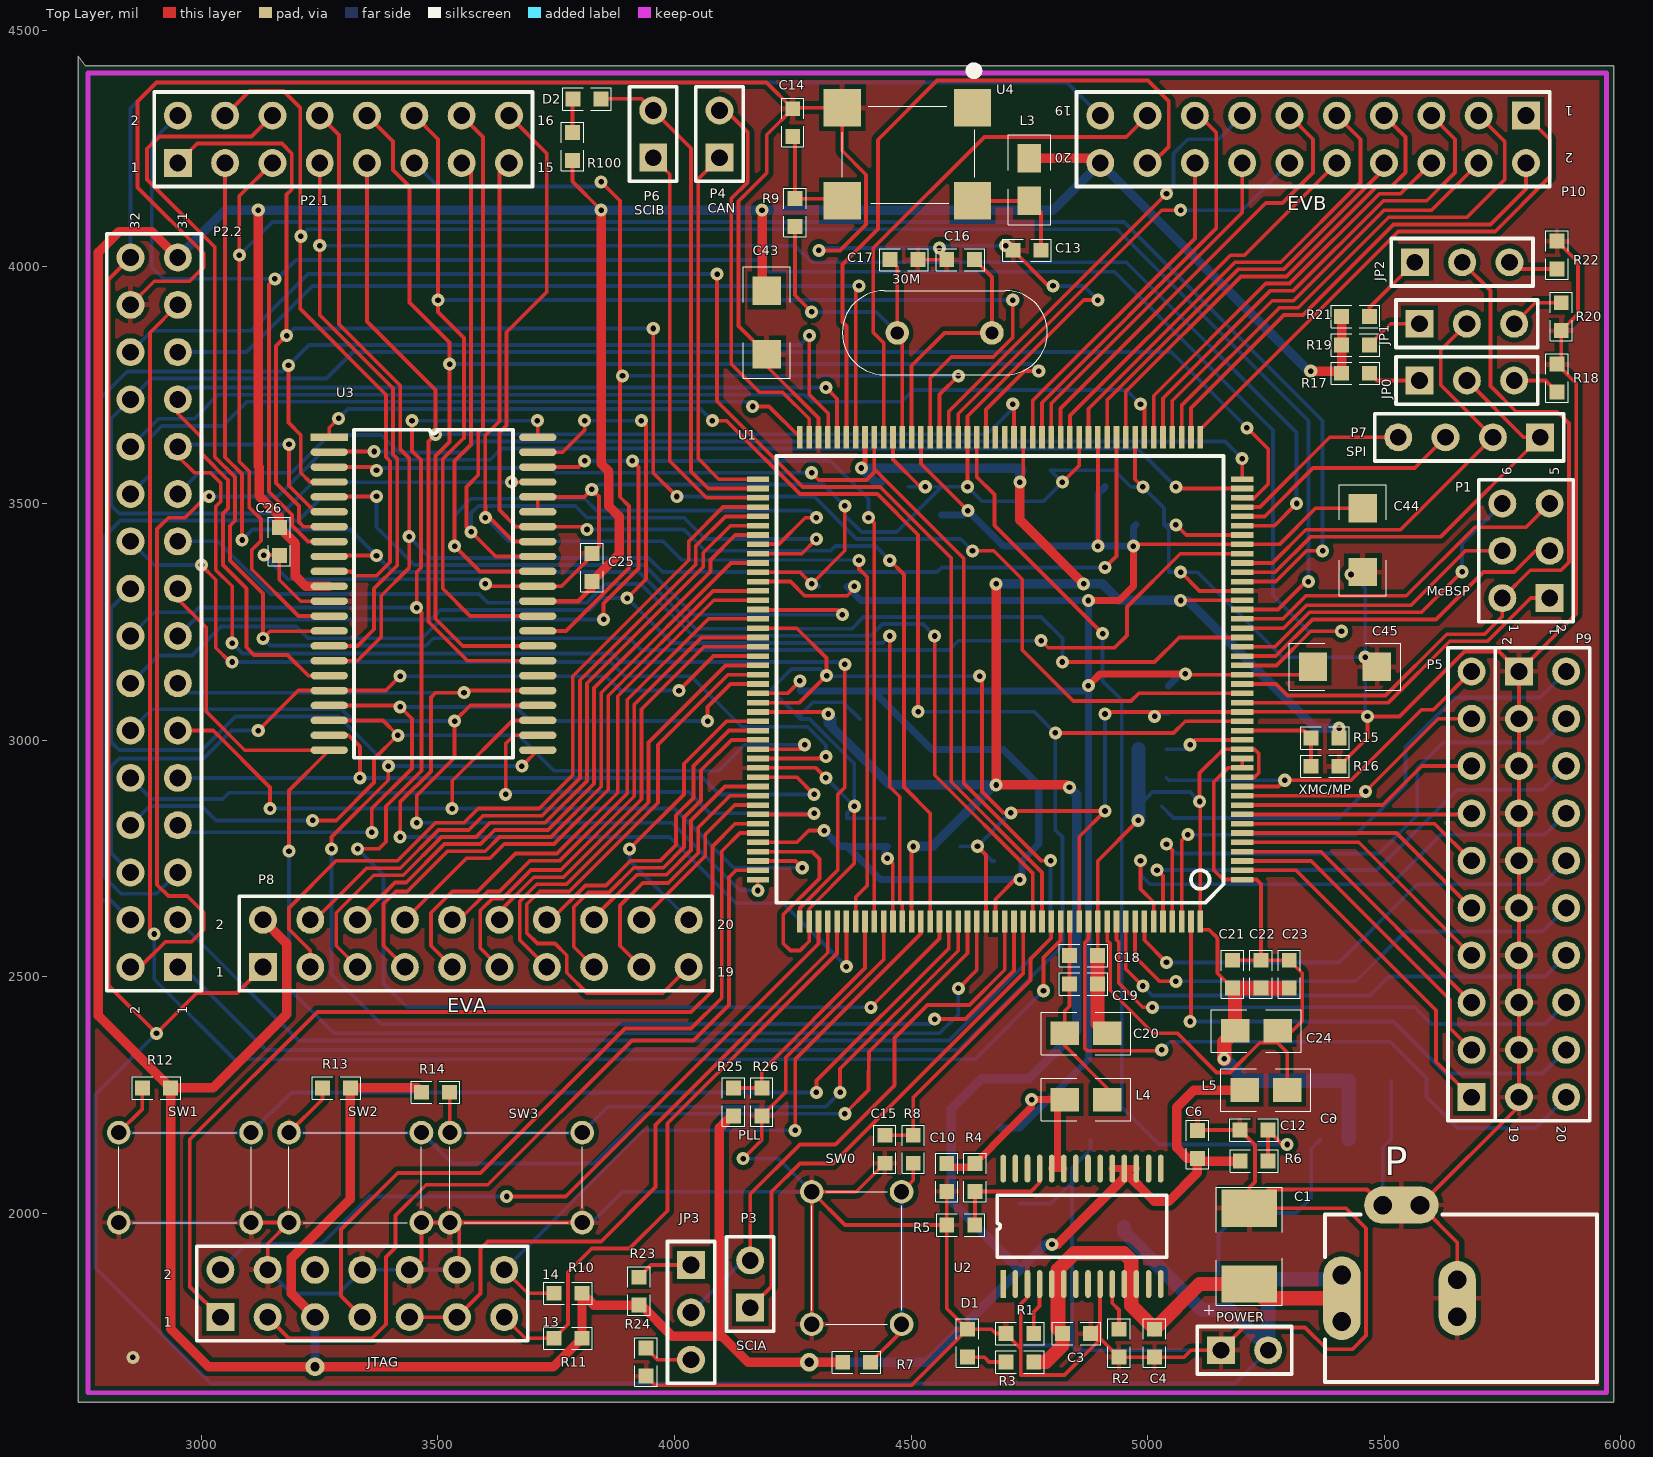
[diagram p0: Top Layer view]
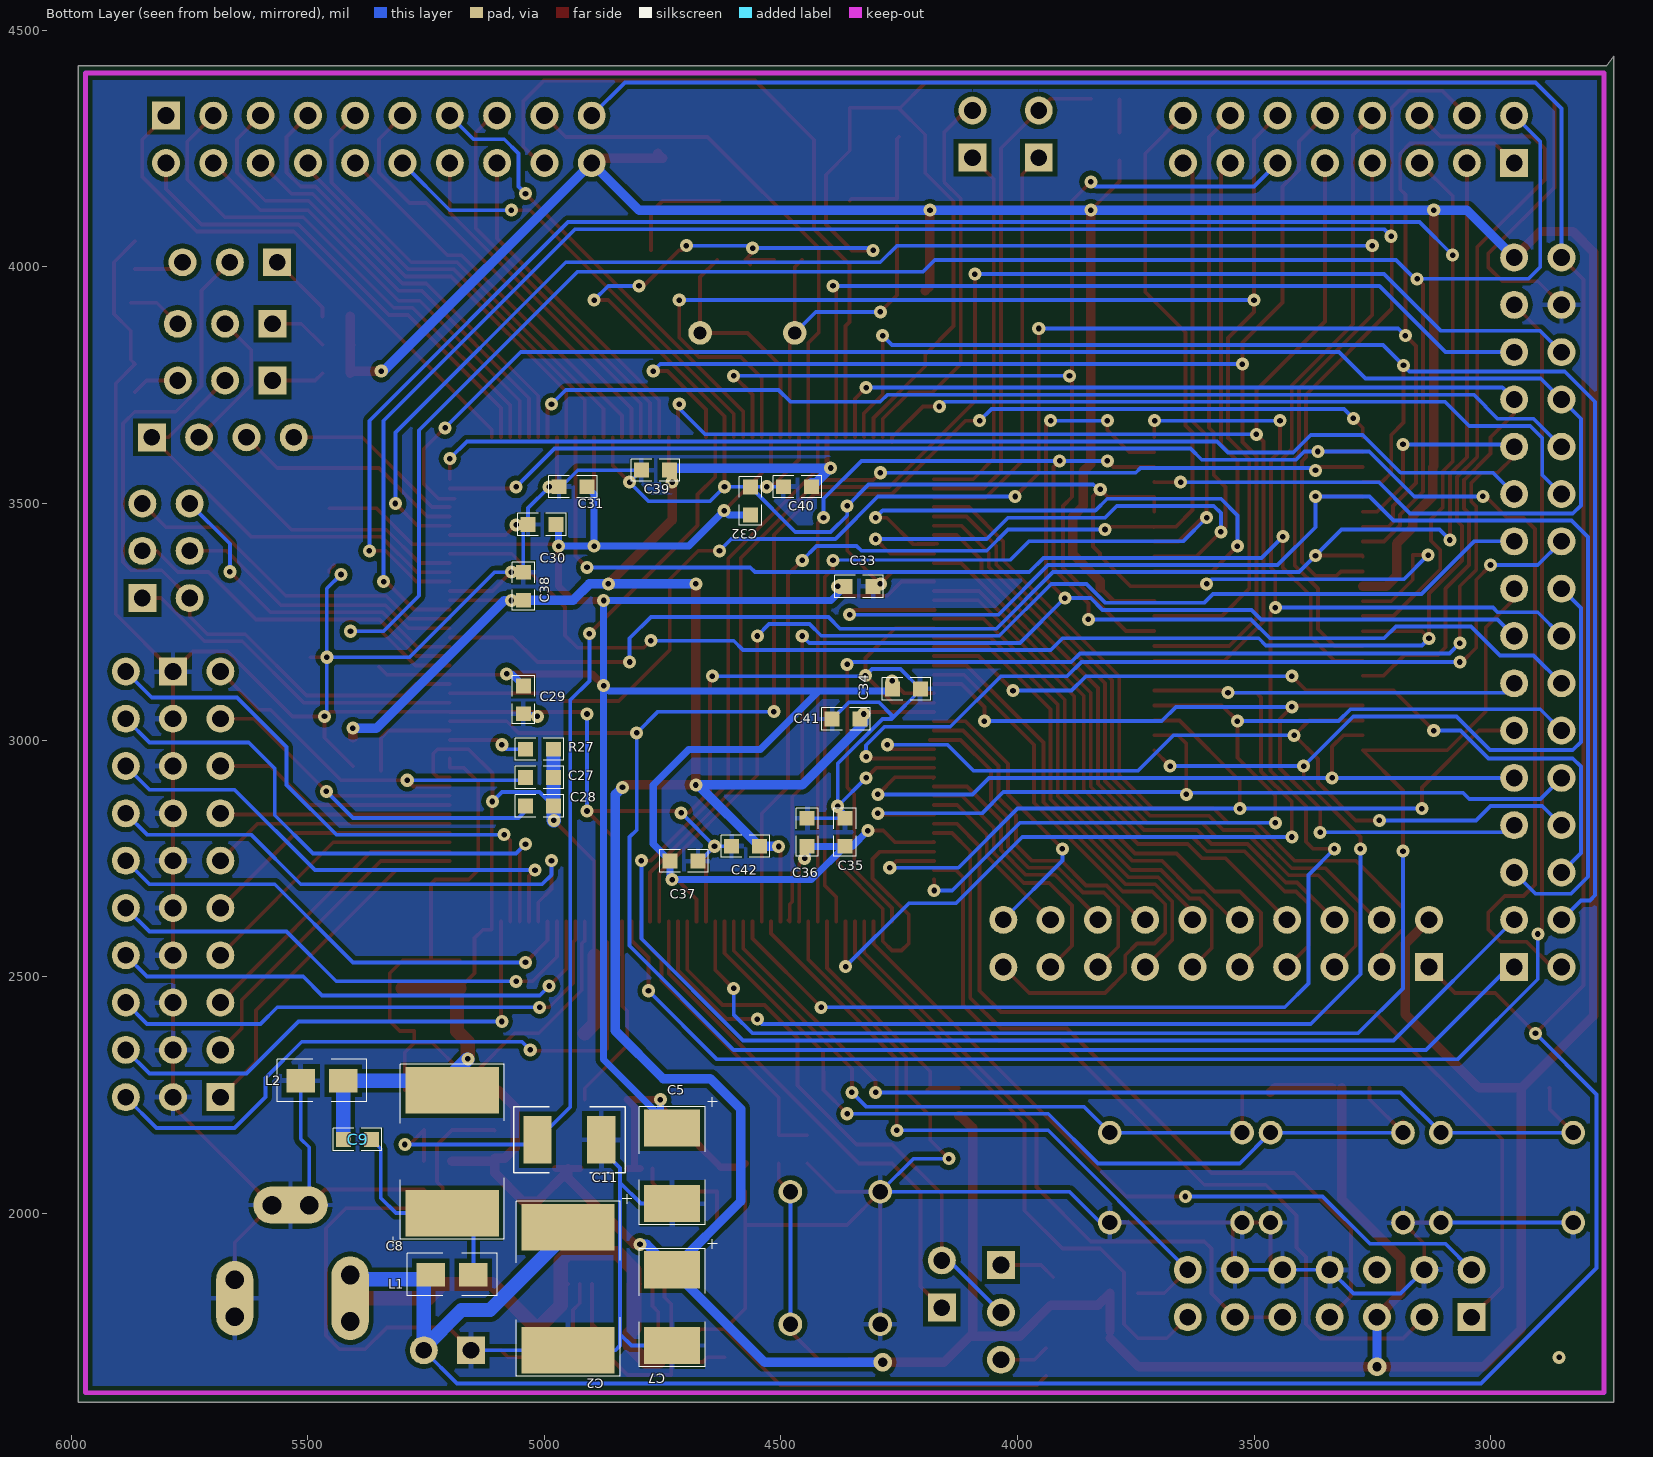
[diagram p1: Bottom Layer view, seen from below]
# Altium PCB MISC76198.PCBDOC (part 1 of 2)
Units mil, origin at the board's own origin, x right, y up, seen from the top; angles counter-clockwise.
Board outline 3245 x 2845 mil, 2 copper layers (Top Layer, Bottom Layer); 107 components, 158 nets, 601 pads, 196 vias.

## Layer stack, top to bottom (the 12.6 mil dielectric is the usual default, probably not edited)
Top Layer: signal copper 1.4
Dielectric: dielectric 12.6, FR-4, Dk 4.8
Bottom Layer: signal copper 1.4

## Board outline
2755,4425 5985,4425 5985,1600 2740,1600 2740,4445

## Design rules (kind name [scope] priority, off if disabled: settings)
Clearance [All] p1: gap=7
ComponentClearance [All] p1: gap=10 collisioncheckmode=0
PolygonConnect [All] p1: connectstyle=Relief reliefconductorwidth=10 reliefentries=4 polygonreliefangle="90 Angle"
RoutingVias [All] p1: holewidth=11.81 width=27.56 viastyle="Through Hole" minholewidth=11 minwidth=27 maxholewidth=39.37 maxwidth=39.37
SolderMaskExpansion [All] p1: expansion=4
TestPointUsage [All] p1: valid=0 allowmultiple=FALSE
Testpoint [All] p1: side=15 testpointundercomponent=TRUE minsize=40 maxsize=100 preferedsize=60 minholesize=0 maxholesize=40 preferedholesize=32 testpointgrid=1 style=1023 order=-539222988
Width Width_2 [InNet('3.3V')] p1: maxlimit=30 minlimit=8 preferedwidth=10 toplayer_prefwidth=8 bottomlayer_prefwidth=20 minimp=50.000000 maximp=50.000000 favimp=50.000000
Width Width_1 [InNet('1.8V')] p2: maxlimit=30 minlimit=8 preferedwidth=10 toplayer_prefwidth=8 bottomlayer_prefwidth=15 minimp=50.000000 maximp=50.000000 favimp=50.000000
Width [All] p3: maxlimit=39.37 minlimit=8 preferedwidth=10 toplayer_prefwidth=8 bottomlayer_prefwidth=8 minimp=50.000000 maximp=50.000000 favimp=50.000000
17 further rules are at their usual default settings.

## Components (designator, comment, footprint, x,y, rotation, side; value= is the part's Value field where it differs from the comment)
30M "XTAL" TXAL 4570,3900 r90 top
C1 "Cap Pol1" C2 5375,1810 r90 top
C2 "Cap Pol1" C1 5035,1910 r270 bottom
C3 "Cap" 0603 4895,1750 r0 top
C4 "Cap" 0603 5010,1770 r90 top
C5 "Cap Pol1" C2 4890,2220 r270 bottom
C6 "Cap" 0603 5110,2100 r270 top
C7 "Cap Pol1" c2 4890,1920 r270 bottom
C8 "Cap Pol1" C1 5110,2060 r90 bottom
C9 "Cap" 0603 5350,2160 r180 bottom
C10 "Cap" 0603 4580,2030 r270 top
C11 "Cap Pol1" 1210 4950,2160 r180 bottom
C12 "Cap" 0603 5270,2180 r0 top
C13 "Cap" 0603 4790,4040 r0 top
C14 "Cap" 0603 4254.56,4260 r270 top
C15 "Cap" 0603 4440,2180 r90 top
C16 "Cap Semi" 0603 4650,4020 r0 top
C17 "Cap Semi" 0603 4530,4020 r0 top
C18 "Cap Semi" 0603 4819.61,2540 r180 top
C19 "Cap Semi" 0603 4819.61,2480 r180 top
C20 "Cap Pol1" 0805 4930,2380 r0 top
C21 "Cap Semi" 0603 5175,2550 r90 top
C22 "Cap Semi" 0603 5235,2550 r90 top
C23 "Cap Semi" 0603 5295,2550 r90 top
C24 "Cap Pol1" 0805 5170,2385 r180 top
C25 "Cap" 0603 3830,3320 r270 top
C26 "Cap" 0603 3160,3465 r90 top
C27 "Cap" 0603 4965,2925 r180 bottom
C28 "Cap" 0603 4965,2865 r180 bottom
C29 "0.1uF" 0603 5040,3040 r270 bottom
C30 "0.1uF" 0603 4960,3460 r180 bottom
C31 "0.1uF" 0603 4894.88,3540 r180 bottom
C32 "0.1uF" 0603 4560,3460 r270 bottom
C33 "0.1uF" 0603 4380,3320 r0 bottom
C34 "0.1uF" 0603 4280,3103.69 r0 bottom
C35 "0.1uF" 0603 4360,2760 r270 bottom
C36 "0.1uF" 0603 4440,2760 r270 bottom
C37 "0.1uF" 0603 4750,2740 r0 bottom
C38 "0.1uF" 0603 5040,3280 r270 bottom
C39 "0.1uF" 0603 4720,3575 r180 bottom
C40 "0.1uF" 0603 4420,3540 r180 bottom
C41 "0.1uF" 0603 4407.44,3040 r0 bottom
C42 "0.1uF" 0603 4530,2780 r180 bottom
C43 "Cap Pol1" 1206 4200,3900 r270 top
C44 "Cap Pol1" 1206 5460,3440 r270 top
C45 "Cap Pol1" 1206 5400,3160 r0 top
D1 "RED" 0603 4615,1770 r90 top
D2 "RED" 0603 3860,4360 r0 top
JP0 "BOOT0" HDR1X3 5575,3760 r0 top (schematic designator JP2)
JP1 "BOOT1" HDR1X3 5575,3880 r0 top (schematic designator JP3)
JP2 "BOOT2" HDR1X3 5565,4010 r0 top (schematic designator JP4)
JP3 "BOOT3" HDR1X3 4035,1890 r270 top (schematic designator JP5)
JTAG "Header 7X2" HDR2X7 3040,1780 r0 top
L1 "Inductor" 0805 5135,1870 r180 bottom
L2 "Inductor" 0805 5410,2280 r180 bottom
L3 "Inductor" 0805 4750.08,4244.85 r90 top
L4 "Inductor" 0805 4930,2240 r0 top
L5 "Inductor" 0805 5190,2260 r180 top
P "PWR2.5" KLD-0202 5950,1820 r180 top
P1 "MCBSP" HDR2X3 5850,3300 r90 top
P2.1 "Header 8X2" HDR2X8 2950,4220 r0 top
P2.2 "Header 16X2" HDR2X16 2950,2520 r90 top (schematic designator P2.3)
P3 "SCIA" HDR1X2 4160,1800 r90 top
P4 "SCIB" HDR1X2 4095,4231 r90 top
P5 "Header 10" HDR1X10 5685,2245 r90 top
P6 "CAN" HDR1X2 3955,4231 r90 top
P7 "SPI" HDR1X4 5830,3640 r180 top
P8 "Header 10X2" HDR2X10 3130,2520 r0 top
P9 "Header 10X2" HDR2X10 5785,3145 r270 top
P10 "Header 10X2" HDR2X10 5800,4320 r180 top
POWER "Header 2" HDR1X2 5155,1710 r0 top
R1 "Res2" 0603 4775,1750 r0 top
R2 "Res2" 0603 4935,1770 r90 top
R3 "Res2" 0603 4775,1690 r0 top
R4 "Res2" 0603 4640,2030 r270 top
R5 "Res2" 0603 4560,1970 r180 top
R6 "Res2" 0603 5180.39,2105.44 r180 top
R7 "1.5K" 0603 4340,1680 r180 top
R8 "100" 0603 4500,2180 r90 top
R9 "1k" 0603 4250,4160 r90 top
R10 "Res2" 0603 3820,1835 r0 top
R11 "Res2" 0603 3820,1740 r0 top
R12 "Res2" 0603 2860,2260 r180 top
R13 "Res2" 0603 3240,2260 r180 top
R14 "Res2" 0603 3540,2260 r0 top
R15 "10K" 0603 5330,3000 r180 top
R16 "1k" 0603 5330,2940 r180 top
R17 "10K" 0603 5485,3780 r0 top
R18 "2.2K" 0603 5870,3720 r270 top
R19 "10K" 0603 5485,3840 r0 top
R20 "2.2K" 0603 5870,3940 r90 top
R21 "10k" 0603 5485,3900 r0 top
R22 "2.2K" 0603 5870,3980 r270 top
R23 "10k" 0603 3920,1880 r90 top
R24 "2.2K" 0603 3935,1730 r90 top
R25 "10k" 0603 4120,2280 r90 top
R26 "2.2K" 0603 4180,2280 r90 top
R27 "24.9K" 0603 4965,2985 r180 bottom
R100 "Res2" 0603 3780,4300 r90 top
SW0 "KEY4" key 4280,2060 r0 top (schematic designator SW1)
SW1 "KEY4" key 3120,2180 r270 top (schematic designator SW4)
SW2 "KEY4" key 3480,2180 r270 top (schematic designator SW3)
SW3 "KEY4" key 3820,2180 r270 top (schematic designator SW2)
U1 "TMS320F2812" QFP176 5200,2705 r90 top locked
U2 "TPS767D301" TSOP28(0.65mm) 4695,1850 r90 top
U3 "CY7C1041CV    SDRAM" TSOP44(0.8mm) 3270,3640 r0 top
U4 "30M" CRYSTAL1 4630,4140 r180 top

## Footprints (in the part's own frame and the unit in brackets; to place one, negate y for a bottom-side part, rotate by r counter-clockwise, add the part's x,y. Pads: shape width x height; smd on the part's side, far side on the other; paste and mask are expansions set on the pad)
0603 [mm]
  rect 0.8x0.8 smd: 1(-1.895,-0.116) 2(-0.395,-0.116)
  silkscreen extent -2.45,-0.72 0.15,0.48
0805 [mil]
  rect 60x50 smd: 1(-105.15,-0.08) 2(-15.15,-0.08)
  silkscreen extent -155,-45 35,45
1206 [mil]
  rect 60x60 smd: 1(-50.17,-5) 2(84.83,-5)
  silkscreen extent -100,-55 135,45
1210 [mil]
  rect 60x100 smd: 1(-64.65,-5.12) 2(70.35,-5.12)
  silkscreen extent -115,-75 120,65
C1 [mm]
  rect 2.5x5 smd: 1(-1.524,2.159) 2(5.08,2.159)
  silkscreen extent -3.3,-0.64 6.48,5.59
C2 [mm]
  rect 2x3 smd: 1(1.016,4.064) 2(5.08,4.064)
  silkscreen extent -0.64,2.29 6.22,6.48
c2 [mm]
  rect 2x3 smd: 1(1.016,4.064) 2(5.08,4.064)
  silkscreen extent -0.63,2.29 6.22,6.48
CRYSTAL1 [mm]
  rect 2x2 smd: 1(0,-5) 2(7,-5) 3(7,0) 4(0,0)
  silkscreen extent -0.27,-7.18 6.98,0.13
HDR1X2 [mm] "Connector; Header; 2 Position"
  rect 1.5x1.5 hole 0.9: 1(0,0)
  round 1.5 hole 0.9: 2(2.54,0)
  silkscreen extent -1.27,-1.27 3.81,1.27
HDR1X3 [mm] "Connector; Header; 3 Position"
  rect 1.5x1.5 hole 0.9: 1(0,0)
  round 1.5 hole 0.9: 2(2.54,0) 3(5.08,0)
  silkscreen extent -1.27,-1.27 6.35,1.27
HDR1X4 [mm] "Connector; Header; 4 Position"
  rect 1.5x1.5 hole 0.9: 1(0,0)
  round 1.5 hole 0.9: 2(2.54,0) 3(5.08,0) 4(7.62,0)
  silkscreen extent -1.27,-1.27 8.89,1.27
HDR1X10 [mm] "Connector; Header; 10 Position"
  rect 1.5x1.5 hole 0.9: 1(0,0)
  round 1.5 hole 0.9: 2(2.54,0) 3(5.08,0) 4(7.62,0) 5(10.16,0) 6(12.7,0) 7(15.24,0) 8(17.78,0) 9(20.32,0) 10(22.86,0)
  silkscreen extent -1.27,-1.27 24.13,1.27
HDR2X3 [mm] "Connector; Header; 3x2 Position"
  rect 1.5x1.5 hole 0.9: 1(0,0)
  round 1.5 hole 0.9: 2(0,2.54) 3(2.54,0) 4(2.54,2.54) 5(5.08,0) 6(5.08,2.54)
  silkscreen extent -1.27,-1.27 6.35,3.81
HDR2X7 [mm] "Connector; Header; 7x2 Position"
  rect 1.5x1.5 hole 0.9: 1(0,0)
  round 1.5 hole 0.9: 2(0,2.54) 3(2.54,0) 4(2.54,2.54) 5(5.08,0) 6(5.08,2.54) 7(7.62,0) 8(7.62,2.54) 9(10.16,0) 10(10.16,2.54) 11(12.7,0) 12(12.7,2.54) 13(15.24,0) 14(15.24,2.54)
  silkscreen extent -1.27,-1.27 16.51,3.81
HDR2X8 [mm] "Connector; Header; 8x2 Position"
  rect 1.5x1.5 hole 0.9: 1(0,0)
  round 1.5 hole 0.9: 2(0,2.54) 3(2.54,0) 4(2.54,2.54) 5(5.08,0) 6(5.08,2.54) 7(7.62,0) 8(7.62,2.54) 9(10.16,0) 10(10.16,2.54) 11(12.7,0) 12(12.7,2.54) 13(15.24,0) 14(15.24,2.54) 15(17.78,0) 16(17.78,2.54)
  silkscreen extent -1.27,-1.27 19.05,3.81
HDR2X10 [mm] "Connector; Header; 10x2 Position"
  rect 1.5x1.5 hole 0.9: 1(0,0)
  round 1.5 hole 0.9: 2(0,2.54) 3(2.54,0) 4(2.54,2.54) 5(5.08,0) 6(5.08,2.54) 7(7.62,0) 8(7.62,2.54) 9(10.16,0) 10(10.16,2.54) 11(12.7,0) 12(12.7,2.54) 13(15.24,0) 14(15.24,2.54) 15(17.78,0) 16(17.78,2.54) 17(20.32,0) 18(20.32,2.54) 19(22.86,0) 20(22.86,2.54)
  silkscreen extent -1.27,-1.27 24.13,3.81
HDR2X16 [mm] "Connector; Header; 16x2 Position"
  rect 1.5x1.5 hole 0.9: 1(0,0)
  round 1.5 hole 0.9: 2(0,2.54) 3(2.54,0) 4(2.54,2.54) 5(5.08,0) 6(5.08,2.54) 7(7.62,0) 8(7.62,2.54) 9(10.16,0) 10(10.16,2.54) 11(12.7,0) 12(12.7,2.54) 13(15.24,0) 14(15.24,2.54) 15(17.78,0) 16(17.78,2.54) 17(20.32,0) 18(20.32,2.54) 19(22.86,0) 20(22.86,2.54) 21(25.4,0) 22(25.4,2.54) 23(27.94,0) 24(27.94,2.54) 25(30.48,0) 26(30.48,2.54) 27(33.02,0) 28(33.02,2.54) 29(35.56,0) 30(35.56,2.54) 31(38.1,0) 32(38.1,2.54)
  silkscreen extent -1.27,-1.27 39.37,3.81
key [mil]
  round 50 hole 32: 1(10,-15) 2(10,-295) 3(200,-15) 4(200,-295)
  silkscreen extent 10,-295 200,-15
KLD-0202 [mm] "DC Power Jack, 2.5mm, KLD Series, PCB Mount"
  oval 2x4.5 all layers, no hole: 1(13.7,0)
  round 1.5 hole 1: 1A(13.7,-1.25) 1B(13.7,1.25) 2A(7.5,-1) 2B(7.5,1) 3A(9.5,-5) 3B(11.5,-5)
  oval 2x4 all layers, no hole: 2(7.5,0)
  oval 4x2 all layers, no hole: 3(10.5,-5)
  silkscreen extent 0,-4.5 14.6,4.5
QFP176 [mm]
  rect 0.3x1.2 smd: 1(0,0) 2(0.5,0) 3(1,0) 4(1.5,0) 5(2,0) 6(2.5,0) 7(3,0) 8(3.5,0) 9(4,0) 10(4.5,0) 11(5,0) 12(5.5,0) 13(6,0) 14(6.5,0) 15(7,0) 16(7.5,0) 17(8,0) 18(8.5,0) 19(9,0) 20(9.5,0) 21(10,0) 22(10.5,0) 23(11,0) 24(11.5,0) 25(12,0) 26(12.5,0) 27(13,0) 28(13.5,0) 29(14,0) 30(14.5,0) 31(15,0) 32(15.5,0) 33(16,0) 34(16.5,0) 35(17,0) 36(17.5,0) 37(18,0) 38(18.5,0) 39(19,0) 40(19.5,0) 41(20,0) 42(20.5,0) 43(21,0) 44(21.5,0) 89(21.5,26) 90(21,26) 91(20.5,26) 92(20,26) 93(19.5,26) 94(19,26) 95(18.5,26) 96(18,26) 97(17.5,26) 98(17,26) 99(16.5,26) 100(16,26) 101(15.5,26) 102(15,26) 103(14.5,26) 104(14,26) 105(13.5,26) 106(13,26) 107(12.5,26) 108(12,26) 109(11.5,26) 110(11,26) 111(10.5,26) 112(10,26) 113(9.5,26) 114(9,26) 115(8.5,26) 116(8,26) 117(7.5,26) 118(7,26) 119(6.5,26) 120(6,26) 121(5.5,26) 122(5,26) 123(4.5,26) 124(4,26) 125(3.5,26) 126(3,26) 127(2.5,26) 128(2,26) 129(1.5,26) 130(1,26) 131(0.5,26) 132(0,26)
  rect 1.2x0.3 smd: 45(23.75,2.25) 46(23.75,2.75) 47(23.75,3.25) 48(23.75,3.75) 49(23.75,4.25) 50(23.75,4.75) 51(23.75,5.25) 52(23.75,5.75) 53(23.75,6.25) 54(23.75,6.75) 55(23.75,7.25) 56(23.75,7.75) 57(23.75,8.25) 58(23.75,8.75) 59(23.75,9.25) 60(23.75,9.75) 61(23.75,10.25) 62(23.75,10.75) 63(23.75,11.25) 64(23.75,11.75) 65(23.75,12.25) 66(23.75,12.75) 67(23.75,13.25) 68(23.75,13.75) 69(23.75,14.25) 70(23.75,14.75) 71(23.75,15.25) 72(23.75,15.75) 73(23.75,16.25) 74(23.75,16.75) 75(23.75,17.25) 76(23.75,17.75) 77(23.75,18.25) 78(23.75,18.75) 79(23.75,19.25) 80(23.75,19.75) 81(23.75,20.25) 82(23.75,20.75) 83(23.75,21.25) 84(23.75,21.75) 85(23.75,22.25) 86(23.75,22.75) 87(23.75,23.25) 88(23.75,23.75) 133(-2.25,23.75) 134(-2.25,23.25) 135(-2.25,22.75) 136(-2.25,22.25) 137(-2.25,21.75) 138(-2.25,21.25) 139(-2.25,20.75) 140(-2.25,20.25) 141(-2.25,19.75) 142(-2.25,19.25) 143(-2.25,18.75) 144(-2.25,18.25) 145(-2.25,17.75) 146(-2.25,17.25) 147(-2.25,16.75) 148(-2.25,16.25) 149(-2.25,15.75) 150(-2.25,15.25) 151(-2.25,14.75) 152(-2.25,14.25) 153(-2.25,13.75) 154(-2.25,13.25) 155(-2.25,12.75) 156(-2.25,12.25) 157(-2.25,11.75) 158(-2.25,11.25) 159(-2.25,10.75) 160(-2.25,10.25) 161(-2.25,9.75) 162(-2.25,9.25) 163(-2.25,8.75) 164(-2.25,8.25) 165(-2.25,7.75) 166(-2.25,7.25) 167(-2.25,6.75) 168(-2.25,6.25) 169(-2.25,5.75) 170(-2.25,5.25) 171(-2.25,4.75) 172(-2.25,4.25) 173(-2.25,3.75) 174(-2.25,3.25) 175(-2.25,2.75) 176(-2.25,2.25)
  silkscreen extent -1.25,1 22.75,25
TSOP28(0.65mm) [mm]
  rect 1.5x0.3 smd: 1(0,0)
  oval 1.5x0.3 smd: 2(0,-0.65) 3(0,-1.3) 4(0,-1.95) 5(0,-2.6) 6(0,-3.25) 7(0,-3.9) 8(0,-4.55) 9(0,-5.2) 10(0,-5.85) 11(0,-6.5) 12(0,-7.15) 13(0,-7.8) 14(0,-8.45) 15(6.2,-8.45) 16(6.2,-7.8) 17(6.2,-7.15) 18(6.2,-6.5) 19(6.2,-5.85) 20(6.2,-5.2) 21(6.2,-4.55) 22(6.2,-3.9) 23(6.2,-3.25) 24(6.2,-2.6) 25(6.2,-1.95) 26(6.2,-1.3) 27(6.2,-0.65) 28(6.2,0)
  silkscreen extent 1.43,-8.78 4.76,0.33
TSOP44(0.8mm) [mm]
  rect 2x0.4 smd: 1(0,0)
  oval 2x0.4 smd: 2(0,-0.8) 3(0,-1.6) 4(0,-2.4) 5(0,-3.2) 6(0,-4) 7(0,-4.8) 8(0,-5.6) 9(0,-6.4) 10(0,-7.2) 11(0,-8) 12(0,-8.8) 13(0,-9.6) 14(0,-10.4) 15(0,-11.2) 16(0,-12) 17(0,-12.8) 18(0,-13.6) 19(0,-14.4) 20(0,-15.2) 21(0,-16) 22(0,-16.8) 23(11.2,-16.8) 24(11.2,-16) 25(11.2,-15.2) 26(11.2,-14.4) 27(11.2,-13.6) 28(11.2,-12.8) 29(11.2,-12) 30(11.2,-11.2) 31(11.2,-10.4) 32(11.2,-9.6) 33(11.2,-8.8) 34(11.2,-8) 35(11.2,-7.2) 36(11.2,-6.4) 37(11.2,-5.6) 38(11.2,-4.8) 39(11.2,-4) 40(11.2,-3.2) 41(11.2,-2.4) 42(11.2,-1.6) 43(11.2,-0.8) 44(11.2,0)
  silkscreen extent 1.33,-17.2 9.87,0.4
TXAL [mm]
  round 1.27 hole 0.7: 1(-0.997,2.518) 2(-0.997,-2.562)
  silkscreen extent -3.26,-5.54 1.27,5.47

## Part data
30M: "Crystal Oscillator"
C1 C2 C5 C7 C8 C11 C20 C24 C43 C44 C45: "Polarized Capacitor (Radial)"
C3 C4 C9 C10 C12 C13 C14 C15 C25 C26 C27 C28: "Capacitor"
C6: library part "Cap Pol1", "Polarized Capacitor (Radial)"
C16 C17 C18 C19 C21 C22 C23: "Capacitor (Semiconductor SIM Model)"
C29 C30 C31 C32 C33 C34 C35 C36 C37 C38 C39 C40 C41 C42: library part Cap, "Capacitor"
D1 D2: library part HLMA-PG00-N0011, "Subminiature High Performance AlInGaP LED Lamp"
JP0 JP1 JP2 JP3: library part "Header 3", "Header, 3-Pin"
JTAG: "Header, 7-Pin, Dual row"
P: "Low Voltage Power Supply Connector"
P1: library part "Header 3X2", "Header, 3-Pin, Dual row"
P2.1: "Header, 8-Pin, Dual row"
P2.2: "Header, 16-Pin, Dual row"
P3 P4 P6: library part "Header 2", "Header, 2-Pin"
P5: "Header, 10-Pin"
P7: library part "Header 4", "Header, 4-Pin"
P8: library part "Header 20X2", "Header, 20-Pin, Dual row"
P9 P10: "Header, 10-Pin, Dual row"
POWER: "Header, 2-Pin"
R1 R2 R3 R4 R5 R6 R10 R11 R12 R13 R14 R100: "Resistor"
R7 R8 R9 R15 R16 R17 R18 R19 R20 R21 R22 R23 R24 R25 R26 R27: library part Res2, "Resistor"
U2: library part TPS73HD301
U3: library part CY7C1041CV

## Via types
v1: diameter 27.56, hole 11.81, Top Layer to Bottom Layer, 194 vias
v2: diameter 39.37, hole 19.68, Top Layer to Bottom Layer, 2 vias

## Nets (pads, with @x,y where several pads share a name; then routed paths per layer and width w, separated by ;. In a path a pad name is that pad's centre, name@x,y a point inside that pad or via, vN(x,y) a via of type N, cw(c..) or ccw(c..) an arc to the next point about the centre after c; other vN are vias at no path point)
1.8V: C5.1 C10.1 C29.1 C30.2 C31.2 C32.2 C33.2 C34.2 C35.2 C36.2 C37.2 C44.1 C45.1 L4.1 R4.1 U1.23 U1.37 U1.56 U1.75 U1.100 U1.112 U1.128 U1.143 U1.154 U2.23 U2.24 | length 7363.4
  Top Layer w8: U1.112@4176.38,3098.7 4238.7,3098.7 v1(4265,3125) ; U1.100@4176.38,3334.92 4245.08,3334.92 4275,3305 4365,3305 v1@4380,3320 ; U1.128@4177.64,2785 U1.128@4176.38,2783.74 4258.74,2783.74 4283.66,2808.66 v1(4316.34,2808.66) ; v1(4450,2750) 4461.22,2738.78 4461.22,2617.01 U1.143@4461.81,2616.42 ; U1.75@4520.87,3640.04 4520.87,3584.13 v1(4620,3485) ; U1.154@4678.35,2616.42 4678.35,2663.35 4720,2705 v1(4730,2705) ; L4.1@4824.77,2240 L4.1@4824.85,2239.92 ; 4894.88,3425.12 U1.56@4894.88,3640.04 4895,3639.92 v1(4895,3410) ; v1(4970,3410) 4973.66,3413.66 5278.66,3413.66 5355.17,3490.17 C44.1@5455,3490.17 ; v1(5080,3140) 5081.93,3138.07 5332.9,3138.07 C45.1@5349.83,3155
  Top Layer w15: C10.1@4575.44,2104.61 4583.11,2096.94 4627.77,2096.94 R4.1@4635.44,2104.61 4671.67,2140.84 ; 4671.67,2141.67 4755,2225 v1(4755,2240) ; v1@4755.08,2239.92 L4.1@4824.85,2239.92 4810,2225.07 4810,2094.09 ; U2.24@4797.36,2094.09 U2.23@4822.95,2094.09 ; v1(4875,3115) 4900,3140 v1(5080,3140) ; v1(4875,3295) 4940,3295 4970,3325 v1(4970,3410)
  Bottom Layer w15: v1@4265.44,3124.45 C34.2@4266.09,3123.8 ; C34.2@4266.09,3123.91 4266.09,3103.69 4863.69,3103.69 v1(4875,3115) ; v1(4316.34,2808.66) 4349.45,2775.55 C35.2@4364.56,2775.55 4435.11,2705 v1(4730,2705) ; C33.2@4364.45,3324.56 4394.01,3295 v1(4875,3295) 4875,2325 C5.1@4730,2180 ; C35.2@4365.11,2775 C36.2@4450,2775 ; 4420,3103.69 4543.69,2980 4695,2980 4770,2905 4770,2780.11 C37.2@4734.45,2744.56 v1@4734.45,2709.45 ; C36.2@4444.56,2775.55 4444.56,2755.44 v1(4450,2750) ; C32.2@4564.56,3475.55 4610.55,3475.55 v1(4620,3485) 4695,3410 v1(4970,3410) 4970,3449.89 C30.2@4975.55,3455.44 ; C5.1@4688,2180 C5.1@4730,2180 ; C5.1@4726.28,2183.72 C5.1@4730,2180 ; C5.1@4755,2205 v1(4755,2240) ; v1(4895,3410) 4895,3520.01 C31.2@4910.43,3535.44 ; C29.1@5044.56,3114.61 5069.95,3140 v1(5080,3140)
  other v1: 4380,3325
3.3V: C6.2 C7.1 C25.2 C26.2 C38.2 C39.2 C40.2 C41.1 C42.2 C43.1 JTAG.5 L3.2 L5.2 P2.2.31 P8.2 P10.20 R6.2 R7.2 R10.2 R11.2 R12.1 R13.1 R14.1 R15.1 R17.1 R19.1 R21.1 R23.1 R25.1 R100.1 U1.31 U1.64 U1.81 U1.114 U1.145 U2.17 U2.18 U2.19 U3.11 U3.33 | length 17306.8
  Top Layer w8: R100.1@3784.56,4225.39 3784.56,4180.44 v1(3845,4120) ; U1.114@4176.38,3059.33 4319.33,3059.33 v1(4325,3055) ; U1.145@4501.18,2616.42 4501.18,2771.18 v1(4505,2775) ; v1(4730,3545) 4737.4,3552.4 U1.64@4737.4,3640.04 ; v1@5070.55,3295.55 U1.31@5200,3295.55
  Top Layer w10: U3.33@3710.94,3293.54 3796.98,3293.54 C25.2@3825.44,3322 ; v1(4395,3575) 4402.76,3582.76 U1.81@4402.76,3640.04
  Top Layer w15: U2.19@4925.32,2094.09 U2.17@4976.5,2094.09
  Top Layer w20: 2782,4031 2782,2417.17 R12.1@2934.61,2264.56 ; 2782.68,4031.68 2826,4075 2895,4075 P2.2.31@2950,4020 ; v1(3120,4120) 3120,3578.78 3121.78,3577 3121.78,3516.02 3164.56,3473.25 C26.2@3164.56,3449.45 3198.63,3415.38 3198.63,3346.66 3220.25,3325.04 U3.11@3270,3325.04 ; P8.2@3130,2620 3180,2570 3180,2420 3024.56,2264.56 R12.1@2934.61,2264.56 ; JTAG.5@3240,1780 3190,1830 3190,1905 3314.61,2029.61 R13.1@3314.61,2264.56 ; 3334.61,2264.56 3456.27,2264.56 R14.1@3465.39,2255.44 ; R11.2@3804.45,1735.44 3744.01,1675 3015,1675 2934.61,1755.39 R12.1@2934.61,2264.56 ; R11.2@3804.45,1750.44 R10.2@3804.45,1830.44 3829.5,1805.39 R23.1@3924.56,1805.39 ; C25.2@3825.44,3322 C25.2@3825.44,3335.55 3882.78,3392.89 3882.78,3472.76 3861.22,3494.32 3861.22,3567.33 3845,3583.55 v1(3845,4120) ; R23.1@3929.61,1805.39 3995,1740 4100,1740 ; R25.1@4124.56,2205.39 4120.39,2205.39 4095,2180 4095,1745 4155.44,1684.56 R7.2@4355.55,1684.56 ; v1(4185,4120) 4185,3960.17 C43.1@4195,3950.17 ; v1(4680,3330) v1(4680,2905) 4830,2905 v1(4835,2900) ; v1(4730,3545) 4730,3465 v1(4865,3330) ; L3.2@4760.46,4240 L3.2@4750.16,4229.7 P10.20@4890.3,4229.7 ; v1(4798,1934) 4809.91,1934 4950.91,2075 U2.18@4950.91,2094.09 ; U2.18@4950.91,2088.19 5014.09,2025 5045,2025 5105.44,2085.44 C6.2@5105.44,2115.55 5084.45,2115.55 5062,2138 5062,2224.08 5098,2260.08 L5.2@5205.15,2260.08 ; C6.2@5114.5,2110 R6.2@5195.94,2110 ; v1(5345,3780) 5405.83,3780 R17.1@5410.39,3775.44 R21.1@5410.39,3895.44 ; R15.1@5404.61,3004.56 5405,3004.95 v1(5405,3025) ; R19.1@5409.5,3834.55 R19.1@5410.39,3835.44
  Bottom Layer w8: v1@4390.44,3570.44 v1(4395,3575)
  Bottom Layer w20: P2.2.31@2950,4020 3050,4120 4800,4120 P10.20@4900,4220 5340,3780 v1(5345,3780) ; v2(3240,1675) JTAG.5@3240,1780 ; v2(4285,1684.56) 4534.56,1684.56 4784,1934 v1(4798,1934) ; C41.1@4325,3034.95 v1(4325,3055) ; C41.1@4332.83,3044.56 4332.83,3027.12 4454.95,2905 v1(4680,2905) ; C40.2@4435.44,3544.45 4425.55,3544.45 v1(4395,3575) C39.2@4730,3575 ; v1(4505,2775) C42.2@4545.11,2775 ; C42.2@4545.55,2775.44 v1@4675.11,2905 ; v1(4680,3330) 4905,3330 4939.45,3295.55 C38.2@5044.56,3295.11 ; C7.1@4730,1880 4585,2025 4585,2220 4649,2284 4749,2284 4850,2385 4850,2885 v1(4835,2900) ; v1(4730,3545) 4730,3564.89 C39.2@4735.55,3570.44 ; C38.2@5044.56,3295.55 5069.45,3295.55 v1(5070,3295) 5085.11,3295 5355.11,3025 v1(5405,3025)
5V: C1.1 C2.1 C3.1 C4.2 L1.1 P2.2.32 P8.1 P10.19 P.1 P.1A P.1B POWER.2 R3.2 U2.5 U2.6 U2.11 U2.12 | length 9567.8
  Top Layer w8: P2.2.32@2850,4020 2803.68,3973.68 2803.68,2481.32 v1(2905,2380) 2990,2465 3075,2465 P8.1@3130,2520 ; U2.5@4797.36,1850 4810.16,1862.8 ; C3.1@4820.39,1745.44 4822.95,1748 U2.6@4822.95,1850 ; 4965.56,1860.94 U2.12@4976.5,1850 ; P.1B@5410.63,1770.79 P.1@5410.63,1820
  Top Layer w10: U2.11@4950.91,1850 4965.56,1850
  Top Layer w30: R3.2@4759.45,1685.44 4785.44,1685.44 4820.39,1720.39 C3.1@4820.39,1745.44 4810,1755.83 4810,1880 4845,1915 4950,1915 4965.56,1899.44 4965.56,1804.44 5014.56,1755.44 C4.2@5014.56,1754.45 5110.11,1850 C1.1@5215,1850 5245,1820 P.1@5410.63,1820
  Bottom Layer w8: P2.2.32@2850,4020 2850,4335 2905,4390 4830,4390 P10.19@4900,4320 ; v1(2905,2380) 2776,2251 2776,1884 3020,1640 5185,1640 POWER.2@5255,1710
  Bottom Layer w30: C2.1@4950,1970 4950,1960 5115,1795 5175,1795 POWER.2@5255,1715 ; L1.1@5240.15,1869.92 5250.07,1860 5410.63,1860 P.1@5410.63,1820 ; POWER.2@5255,1710 L1.1@5255,1855.07
ADCBGREFN: P9.20 U1.164 | length 1425
  Top Layer w8: U1.164@4875.2,2616.42 4875.2,2579.2 4867,2571 4867,2349 4873,2343 5028,2343 v1(5030,2345)
  Bottom Layer w8: v1(5030,2345) 5047.15,2362.15 5512.85,2362.15 5589.47,2285.53 5589.47,2245.53 5655,2180 5820,2180 P9.20@5885,2245
ADCINA0: P9.2 U1.174 | length 1178.7
  Top Layer w8: U1.174@5072.05,2616.42 5072.05,2787.05 v1(5085,2800)
  Bottom Layer w8: v1(5085,2800) 5440,2800 5545,2905 5545,2985 5650,3090 5830,3090 P9.2@5885,3145
ADCINA1: P9.4 U1.173 | length 1198
  Top Layer w8: v1(5040,2780) 5052.36,2767.64 U1.173@5052.36,2616.42
  Bottom Layer w8: v1(5040,2780) 5060,2760 5489,2760 5570,2841 5570,2940 5625,2995 5835,2995 P9.4@5885,3045
ADCINA2: P9.6 U1.172 | length 1070
  Top Layer w8: v1(5020,2725) 5032.68,2712.32 U1.172@5032.68,2616.42
  Bottom Layer w8: v1(5020,2725) 5485,2725 5655,2895 5835,2895 P9.6@5885,2945
ADCINA3: P9.8 U1.171 | length 1140.6
  Top Layer w8: v1(4985,2745) 4985,2685 5012.99,2657.01 U1.171@5012.99,2616.42
  Bottom Layer w8: v1(4985,2745) 4985,2715 5005,2695 5515,2695 5620,2800 5840,2800 P9.8@5885,2845
ADCINA4: P9.10 U1.170 | length 1039.8
  Top Layer w8: U1.170@4993.31,2616.42 4993.31,2576.69 v1(5040,2530)
  Bottom Layer w8: v1(5040,2530) 5405,2530 5570,2695 5835,2695 P9.10@5885,2745
ADCINA5: P9.12 U1.169 | length 1071.7
  Top Layer w8: U1.169@4973.62,2616.42 4973.62,2541.73 5025.36,2490 v1(5060,2490)
  Bottom Layer w8: v1(5060,2490) 5440,2490 5545,2595 5835,2595 P9.12@5885,2645
ADCINA6: P9.14 U1.168 | length 1089.8
  Top Layer w8: U1.168@4953.94,2616.42 4953.94,2516.06 v1(4990,2480)
  Bottom Layer w8: v1(4990,2480) 5010,2460 5470,2460 5510,2500 5840,2500 P9.14@5885,2545
ADCINA7: P9.16 U1.167 | length 1132.6
  Top Layer w8: U1.167@4934.25,2616.42 4934.25,2577.96 4938.94,2573.28 4938.94,2486.06 4990,2435 v1(5010,2435)
  Bottom Layer w8: v1(5010,2435) 5565,2435 5600,2400 5840,2400 P9.16@5885,2445
ADCINB0: P5.1 U1.2 | length 747.3
  Top Layer w8: U1.2@5200,2724.69 5313.92,2724.69 5610,2428.61 5610,2320 P5.1@5685,2245
ADCINB1: P5.2 U1.3 | length 685.8
  Top Layer w8: U1.3@5200,2744.37 5346,2744.37 5640,2450.37 5640,2390 P5.2@5685,2345
ADCINB2: P5.3 U1.4 | length 617.2
  Top Layer w8: U1.4@5200,2764.06 5365.94,2764.06 P5.3@5685,2445
ADCINB3: P5.4 U1.5 | length 583.9
  Top Layer w8: U1.5@5200,2783.74 5446.26,2783.74 P5.4@5685,2545
ADCINB4: P5.5 U1.6 | length 550.6
  Top Layer w8: U1.6@5200,2803.43 5526.57,2803.43 P5.5@5685,2645
ADCINB5: P5.6 U1.7 | length 517.4
  Top Layer w8: U1.7@5200,2823.11 5606.89,2823.11 P5.6@5685,2745
ADCINB6: P5.7 U1.8 | length 485.9
  Top Layer w8: U1.8@5200,2842.8 5682.8,2842.8 P5.7@5685,2845
ADCINB7: P5.8 U1.9 | length 519.2
  Top Layer w8: U1.9@5200,2862.48 5497.06,2862.48 5579.58,2945 P5.8@5685,2945
ADCLO: P9.18 U1.175 | length 1073.4
  Top Layer w8: v1(5090,2405) 5091.73,2406.73 U1.175@5091.73,2616.42
  Bottom Layer w8: v1(5090,2405) 5520,2405 5630,2295 5835,2295 P9.18@5885,2345
ADCREFM: C28.1 P5.9 U1.10 | length 1017.1
  Top Layer w8: U1.10@5200,2882.17 5451.67,2882.17 5614.5,3045 P5.9@5685,3045
  Bottom Layer w8: C28.1@5030,2860 5055,2835 5404.5,2835 v1(5460.92,2891.42)
ADCREFP: C27.1 P5.10 U1.11 | length 838.4
  Top Layer w8: U1.11@5200,2901.85 5276.85,2901.85 v1(5290,2915) 5430,2915 5579.19,3064.19 5604.19,3064.19 P5.10@5685,3145
  Bottom Layer w8: C27.1@5039.61,2920.44 5045.05,2915 v1(5290,2915)
AGND: C8.2 C9.1 C18.1 C19.1 C20.2 C21.1 C22.1 C23.1 C24.2 C27.2 C28.2 L2.2 R27.2 U1.12 U1.15 U1.165 U1.176 | length 2240.9
  Top Layer w8: C18.1@4894.22,2544.56 4894.88,2545.23 4894.88,2744.88 v1(4980,2830) ; C21.1@5179.56,2475.39 5147.78,2507.17 5147.78,2581.22 5130,2599 5111.42,2599 5111.42,2868.58 v1(5110,2870) 5110,2930 5160.59,2980.59 5226,2980.59 5235,2971.59 5235,2930.54 5226,2921.54 U1.12@5200,2921.54
  Top Layer w30: C18.1@4894.22,2544.56 4894.22,2400.56 C20.2@4914.85,2379.92 ; v1(5162,2326) 5162,2361.93 C24.2@5185.15,2385.08 5185.15,2469.8 C21.1@5179.56,2475.39 C23.1@5299.56,2475.39
  Bottom Layer w8: C28.2@4980.55,2860.44 5010.11,2890 5090,2890 v1(5110,2870)
  Bottom Layer w30: v1(4980,2830) 4980.55,2830.55 R27.2@4980.55,2980.44 ; v1@5163.22,2324.78 5195,2293 C8.2@5195,2260 5214.92,2279.92 L2.2@5425.15,2279.92 5425.15,2155.98 C9.1@5424.61,2155.44
C1TRIP: P8.16 U1.122 | length 502.7
  Top Layer w8: P8.16@3830,2620 3830,2625 3920,2715 3982.57,2715 4035,2767.43 4035,2830 4106.85,2901.85 U1.122@4176.38,2901.85
C2TRIP: P8.17 U1.123 | length 583.2
  Top Layer w8: P8.17@3930,2520 3885,2565 3885,2650 3932.9,2697.9 3986.68,2697.9 4050,2761.21 4050,2815 4117.17,2882.17 U1.123@4176.38,2882.17
  Bottom Layer w8: P8.17@3930,2520 P8.17@3930,2535.53
C3TRIP: P8.18 U1.124 | length 387.3
  Top Layer w8: P8.18@3920,2630 P8.18@3930,2620 4065,2755 4065,2800 4127.48,2862.48 U1.124@4176.38,2862.48
C4TIP: P10.14 U1.61 | length 747.1
  Top Layer w8: U1.61@4796.46,3640.04 4796.46,3711.46 5200,4115 P10.14@5200,4220
C5TIP: P10.15 U1.62 | length 857
  Top Layer w8: U1.62@4776.77,3640.04 4776.77,3712.99 5145,4081.21 5145,4285 5110,4320 P10.15@5100,4320
C6TIP: P10.16 U1.63 | length 722
  Top Layer w8: U1.63@4757.09,3640.04 4757.09,3717.09 5100,4060 P10.16@5100,4220
CANRXA: P4.1 U1.89 | length 799.1
  Top Layer w8: P4.1@4095,4231 4050,4186 4050,3595 4093.54,3551.46 U1.89@4176.38,3551.46
CANTXA: P4.2 U1.87 | length 835
  Top Layer w8: P4.2@4095,4331 4108.5,4331 4155,4284.5 4155,4180 4120,4145 4120,3795 4180,3735 4228.79,3735 4284.65,3679.14 U1.87@4284.65,3640.04
CAP1-QEP1: P8.11 U1.106 | length 1075.9
  Top Layer w8: P8.11@3630,2520 3589.47,2560.53 3589.47,2639.47 3615,2665 3636.36,2665 3696.9,2725.54 3759.47,2725.54 3915,2881.07 3915,3075 4056.81,3216.81 U1.106@4176.38,3216.81
CAP2-QEP2: P8.12 U1.107 | length 907
  Top Layer w8: P8.12@3630,2620 3630,2637.43 3702.57,2710 3765.15,2710 3930,2874.85 3930,3065 4062.13,3197.13 U1.107@4176.38,3197.13
CAP3-QEPI1: P8.13 U1.109 | length 946.9
  Top Layer w8: P8.13@3730,2520 3672.77,2577.23 3672.77,2658.98 3708.79,2695 3771.36,2695 3945,2868.64 3945,2995 4107.76,3157.76 U1.109@4176.38,3157.76
CAP4: P10.9 U1.57 | length 995.2
  Top Layer w8: U1.57@4875.2,3640.04 4875.2,3700.2 5185,4010 5281.36,4010 5450,4178.64 5450,4270 P10.9@5400,4320
CAP5: P10.10 U1.59 | length 831.2
  Top Layer w8: U1.59@4835.83,3640.04 4835.83,3685.83 5175,4025 5205,4025 P10.10@5400,4220
CAP6: P10.11 U1.60 | length 942.3
  Top Layer w8: U1.60@4816.14,3640.04 4816.14,3701.14 5250,4135 5285,4135 5350,4200 5350,4270 P10.11@5300,4320
EMU0: JTAG.13 R11.1 U1.137 | length 1299.5
  Top Layer w8: JTAG.13@3640,1780 3684.56,1735.44 R11.1@3745.39,1735.44 3775,1765.05 3775,1875 3825,1925 3905,1925 3985,2005 3985,2190 4343.7,2548.7 U1.137@4343.7,2616.42
EMU1: JTAG.14 R10.1 U1.146 | length 1414.7
  Top Layer w8: JTAG.14@3640,1880 3689.56,1830.44 R10.1@3745.39,1830.44 ; v1(4255,2175) 4255,2325 4520.87,2590.87 U1.146@4520.87,2616.42
  Bottom Layer w8: JTAG.14@3640,1880 3935,2175 v1(4255,2175)